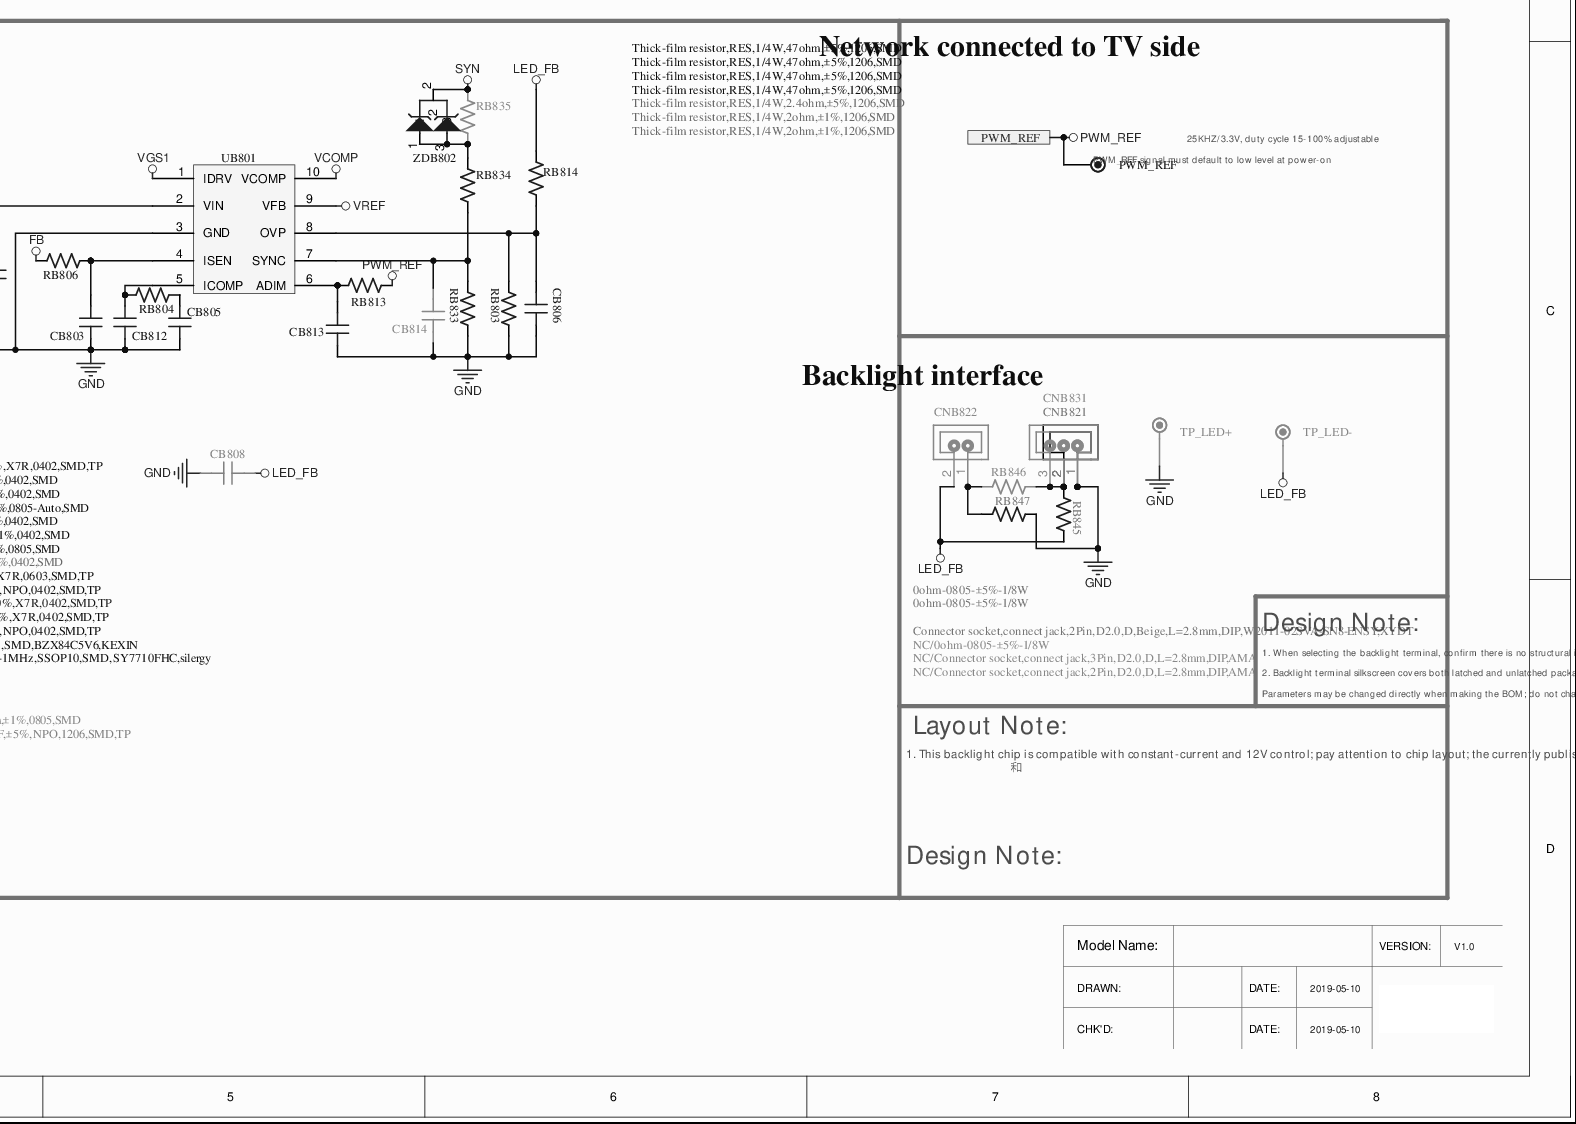
[diagram p0: MISC86372-5.SchDoc, bottom right]
# Altium project MISC86372-32.PrjPCB (part 8 of 8)

## Nets that join several sheets
3V3_STB: MISC86372-8 (6 pins), MISC86372-9 (22 pins), MISC86372-10 (RK3.2 RK13.2), MISC86372-14 (RH104.2 RH106.2), MISC86372-15 (RA35.2), MISC86372-16 (RT1.2)
3V3_TUNER: MISC86372-9 (RF43.1 RF44.1), MISC86372-16 (14 pins)
5V_M: MISC86372-8 (6 pins), MISC86372-10 (RK10.2), MISC86372-12 (RI48.1), MISC86372-13 (FU1.2 RO33.1 RU4.2)
5V_STB: MISC86372-8 (17 pins), MISC86372-10 (RK1.2 RK5.1), MISC86372-12 (RF8.2 RF9.2)
12V: MISC86372-8 (5 pins), MISC86372-11 (CM11.2 QM12.S RM13.1), MISC86372-15 (13 pins), MISC86372-5 (11 pins)
+1.8V_DDR: MISC86372-8 (5 pins), MISC86372-9 (6 pins)
GND: MISC86372-4 (30 pins), MISC86372-8 (32 pins), MISC86372-9 (38 pins), MISC86372-10 (11 pins), MISC86372-11 (15 pins), MISC86372-12 (52 pins), MISC86372-13 (35 pins), MISC86372-14 (37 pins), MISC86372-15 (34 pins), MISC86372-16 (39 pins), MISC86372-5 (41 pins)
PWM_REF: MISC86372-9 (CG201.1 RG61.2 RG61.3), MISC86372-5 (PWM_REF.1 RB813.1)
VDDC_CORE: MISC86372-8 (8 pins), MISC86372-9 (13 pins)
AMP_L_OUT_IC: MISC86372-9 (CF29.1 U1.41), MISC86372-15 (CA32.2 RA3.1)
AMP_MUTE_OUT_IC: MISC86372-9 (U1.90), MISC86372-15 (RA1.1 RA2.2)
AMP_R_OUT_IC: MISC86372-9 (CF30.1 U1.42), MISC86372-15 (CA31.2 RA14.1)
AU_CTRL_IC: MISC86372-9 (U1.53), MISC86372-12 (RI3.1)
AV1_CVBS_IN_IC: MISC86372-9 (U1.31), MISC86372-12 (CI2.2)
AV1_L_IN_IC: MISC86372-9 (U1.37), MISC86372-12 (CI3.1 CI6.1 RI5.2)
AV1_R_IN_IC: MISC86372-9 (U1.38), MISC86372-12 (CI4.1 CI8.1 RI6.2)
CVBS_OUT_IC: MISC86372-9 (U1.33), MISC86372-13 (DO1.K RO1.2 RO2.2 RO3.2)
EPH_DET_IN_IC: MISC86372-9 (U1.58), MISC86372-15 (CA33.2 RA36.1)
HDMI_A_0N_IN_IC: MISC86372-9 (U1.1), MISC86372-14 (JH1.9)
HDMI_A_0P_IN_IC: MISC86372-9 (U1.2), MISC86372-14 (JH1.7)
HDMI_A_1N_IN_IC: MISC86372-9 (U1.3), MISC86372-14 (JH1.6)
HDMI_A_1P_IN_IC: MISC86372-9 (U1.4), MISC86372-14 (JH1.4)
HDMI_A_2N_IN_IC: MISC86372-9 (U1.5), MISC86372-14 (JH1.3)
HDMI_A_2P_IN_IC: MISC86372-9 (U1.6), MISC86372-14 (JH1.1)
HDMI_A_CKN_IN_IC: MISC86372-9 (U1.127), MISC86372-14 (JH1.12)
HDMI_A_CKP_IN_IC: MISC86372-9 (U1.128), MISC86372-14 (JH1.10)
HDMI_A_HPD_OUT_IC: MISC86372-9 (U1.120), MISC86372-14 (RH4.2 RH4.4)
HDMI_A_SCL_IN_IC: MISC86372-9 (U1.107), MISC86372-14 (RH6.2)
HDMI_A_SDA_IO_IC: MISC86372-9 (U1.106), MISC86372-14 (RH5.2)
HDMI_ARC_OUT_IC: MISC86372-9 (U1.125), MISC86372-14 (CH81.2)
HDMI_B_0N_IN_IC: MISC86372-9 (U1.9), MISC86372-14 (JH21.9)
HDMI_B_0P_IN_IC: MISC86372-9 (U1.10), MISC86372-14 (JH21.7)
HDMI_B_1N_IN_IC: MISC86372-9 (U1.11), MISC86372-14 (JH21.6)
HDMI_B_1P_IN_IC: MISC86372-9 (U1.12), MISC86372-14 (JH21.4)
HDMI_B_2N_IN_IC: MISC86372-9 (U1.13), MISC86372-14 (JH21.3)
HDMI_B_2P_IN_IC: MISC86372-9 (U1.14), MISC86372-14 (JH21.1)
HDMI_B_CKN_IN_IC: MISC86372-9 (U1.7), MISC86372-14 (JH21.12)
HDMI_B_CKP_IN_IC: MISC86372-9 (U1.8), MISC86372-14 (JH21.10)
HDMI_B_HPD_OUT_IC: MISC86372-9 (U1.121), MISC86372-14 (RH24.1 RH24.3)
HDMI_B_SCL_IN_IC: MISC86372-9 (U1.116), MISC86372-14 (RH26.2)
HDMI_B_SDA_IO_IC: MISC86372-9 (U1.115), MISC86372-14 (RH25.2)
HDMI_CEC_IO_IC: MISC86372-9 (U1.119), MISC86372-14 (RH83.1)
HDMI_DET: MISC86372-9 (U1.110), MISC86372-14 (RH81.1 RH82.1)
IR_IN_IC: MISC86372-9 (U1.97), MISC86372-10 (CK1.2 RK2.2)
KEY_IN_IC: MISC86372-9 (U1.109), MISC86372-10 (CK3.2 RK4.1)
LED_OUT_IC: MISC86372-9 (U1.92), MISC86372-10 (RK13.1 RK14.2 RK15.2)
LINE_L_OUT_IC: MISC86372-9 (U1.39), MISC86372-13 (CO11.2 RO12.2)
LINE_R_OUT_IC: MISC86372-9 (U1.40), MISC86372-13 (CO14.2 RO15.2)
LVDS_E0N_IC: MISC86372-9 (U1.76), MISC86372-11 (CNW1.19 CNW2.19)
LVDS_E0P_IC: MISC86372-9 (U1.75), MISC86372-11 (CNW1.20 CNW2.20)
LVDS_E1N_IC: MISC86372-9 (U1.74), MISC86372-11 (CNW1.21 CNW2.21)
LVDS_E1P_IC: MISC86372-9 (U1.73), MISC86372-11 (CNW1.22 CNW2.22)
LVDS_E2N_IC: MISC86372-9 (U1.72), MISC86372-11 (CNW1.23 CNW2.23)
LVDS_E2P_IC: MISC86372-9 (U1.71), MISC86372-11 (CNW1.24 CNW2.24)
LVDS_E3N_IC: MISC86372-9 (U1.68), MISC86372-11 (CNW1.29 CNW2.29)
LVDS_E3P_IC: MISC86372-9 (U1.67), MISC86372-11 (CNW1.30 CNW2.30)
LVDS_ECKN_IC: MISC86372-9 (U1.70), MISC86372-11 (CNW1.27 CNW2.27)
LVDS_ECKP_IC: MISC86372-9 (U1.69), MISC86372-11 (CNW1.28 CNW2.28)
LVDS_O0N_IC: MISC86372-9 (U1.89), MISC86372-11 (CNW1.7 CNW2.7)
LVDS_O0P_IC: MISC86372-9 (U1.88), MISC86372-11 (CNW1.8 CNW2.8)
LVDS_O1N_IC: MISC86372-9 (U1.87), MISC86372-11 (CNW1.9 CNW2.9)
LVDS_O1P_IC: MISC86372-9 (U1.86), MISC86372-11 (CNW1.10 CNW2.10)
LVDS_O2N_IC: MISC86372-9 (U1.84), MISC86372-11 (CNW1.11 CNW2.11)
LVDS_O2P_IC: MISC86372-9 (U1.83), MISC86372-11 (CNW1.12 CNW2.12)
LVDS_O3N_IC: MISC86372-9 (U1.80), MISC86372-11 (CNW1.17 CNW2.17)
LVDS_O3P_IC: MISC86372-9 (U1.79), MISC86372-11 (CNW1.18 CNW2.18)
LVDS_OCKN_IC: MISC86372-9 (U1.82), MISC86372-11 (CNW1.15 CNW2.15)
LVDS_OCKP_IC: MISC86372-9 (U1.81), MISC86372-11 (CNW1.16 CNW2.16)
MAIN_SCL_OUT_IC: MISC86372-9 (DK3.K RF43.2 U1.52), MISC86372-16 (RT2.1)
MAIN_SDA_IO_IC: MISC86372-9 (DK2.K RF44.2 U1.51), MISC86372-16 (RT3.1)
PANEL_EN_OUT_IC: MISC86372-9 (U1.93), MISC86372-11 (RM11.1)
POWER_EN_OUT_IC: MISC86372-8 (RM1.1 RM2.1), MISC86372-9 (U1.57)
SPDIF_OUT_IC: MISC86372-9 (U1.94), MISC86372-13 (CO31.2 RO21.1)
TUNER_AGC_OUT_IC: MISC86372-9 (U1.43), MISC86372-16 (CT26.2 RT7.2 RT8.2)
TUNER_IF_N_IN_IC: MISC86372-9 (U1.45), MISC86372-16 (CT12.1)
TUNER_IF_P_IN_IC: MISC86372-9 (U1.44), MISC86372-16 (CT11.1)
UART_RX_IC: MISC86372-9 (U1.104), MISC86372-12 (RF8.1 RF11.1), MISC86372-14 (CD101.K RH105.2 RH106.1)
UART_TX_IC: MISC86372-9 (U1.103), MISC86372-12 (RF9.1 RF10.1), MISC86372-14 (CD102.K RH103.2 RH104.1)
USB0_DM_IO_IC: MISC86372-9 (U1.63), MISC86372-13 (RU1.1)
USB0_DP_IO_IC: MISC86372-9 (U1.64), MISC86372-13 (RU2.1)
USB1_DM_IO_IC: MISC86372-9 (U1.61), MISC86372-13 (RU3.1)
USB1_DP_IO_IC: MISC86372-9 (U1.62), MISC86372-13 (RU5.1)
VGA_HS_IN_IC: MISC86372-9 (U1.25), MISC86372-12 (CV5.2 RV9.2)
VGA_VS_IN_IC: MISC86372-9 (U1.30), MISC86372-12 (CV4.2 RV7.2)
XTAL_OUT: MISC86372-9 (L6.2), MISC86372-16 (UT2.13)
YPP_Pb&B_IN_IC: MISC86372-9 (U1.26), MISC86372-12 (CV3.2)
YPP_Pr&R_IN_IC: MISC86372-9 (U1.29), MISC86372-12 (CV1.2)
YPP_Y&G_IN_IC: MISC86372-9 (U1.27), MISC86372-12 (CV2.2)